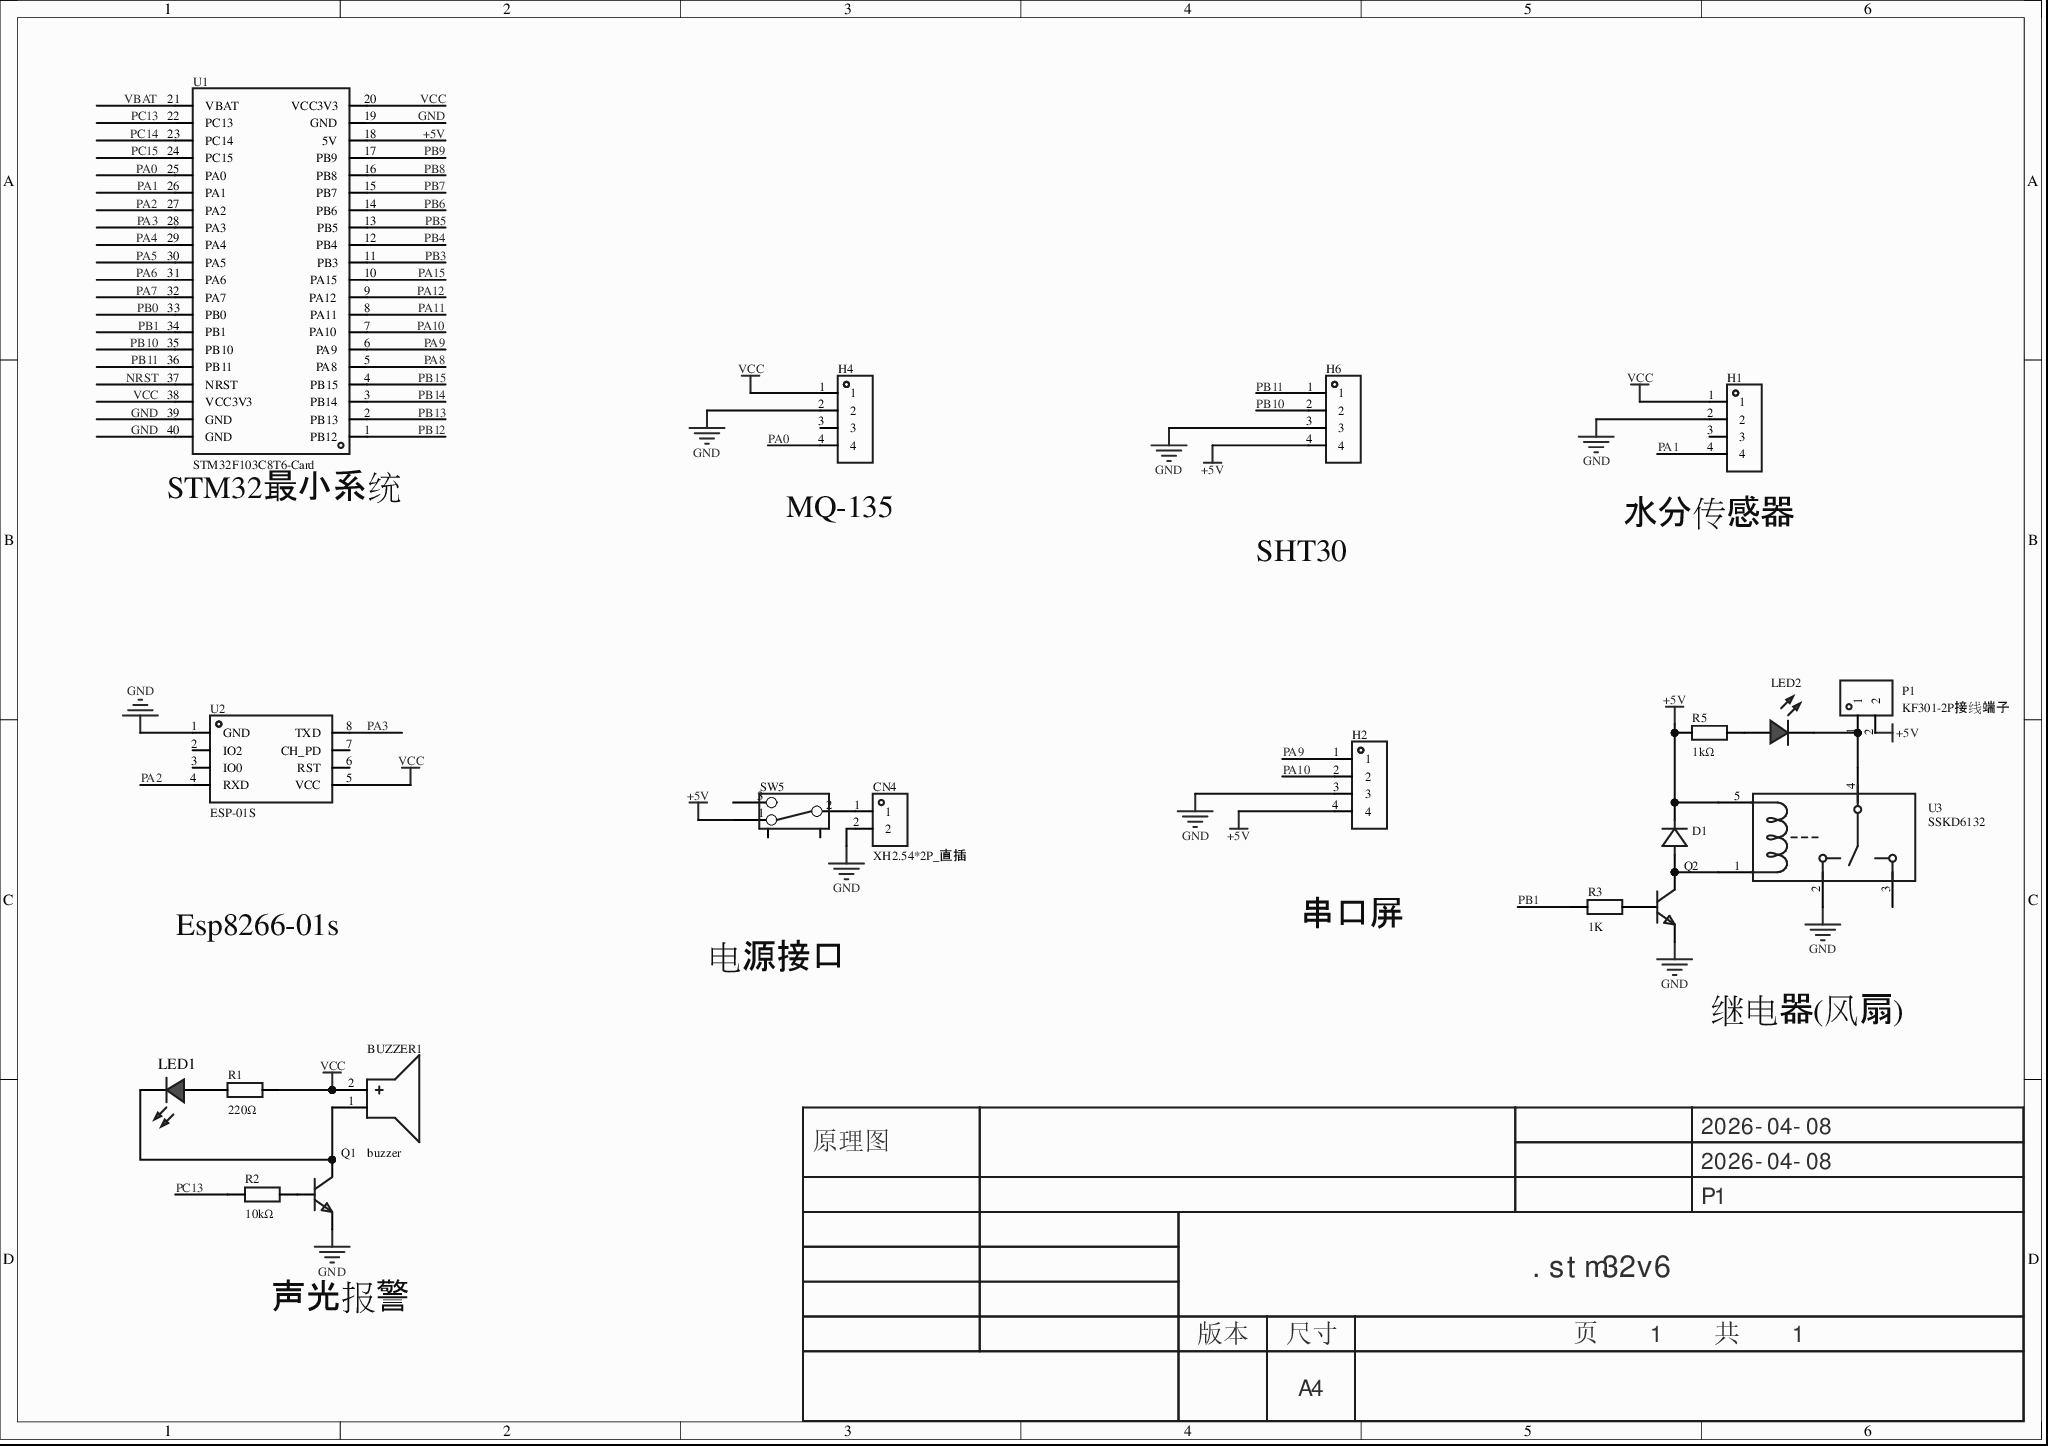
[diagram p0: MISC52093-3.schdoc]
# Altium project MISC52093-2.PrjPcb
1 sheet, 20 parts. Net scope: global (net labels, ports and power ports of the same name join across sheets).
Board file: MISC52093.pcbdoc

## Sheet MISC52093-3.schdoc
size 297 x 209 mm; Version: V1.0; @Project Name: MISC52093; @Page Count: 1; @Update Date: 2026-04-08; @Create Date: 2026-04-08; @Schematic Name: MISC52093; @Page No: 1; @Create Time: 23:22:16; @Update Time: 17:32:40; @Board Name: MISC52093

### Parts
BUZZER1  buzzer  [BUZ-TH_BD12.0-P6.00-D0.9-RD]
CN4  XH2.54*2P_直插  [CONN-TH_2P-P2.50-XH2.54-2P]
D1  (no value)  [SMA_1N4007]
H1  (no value)  [HDR-TH_4P-P2.54-V-F]
H2  (no value)  [HDR-TH_4P-P2.54-V-F]
H4  (no value)  [HDR-TH_4P-P2.54-V-F]
H6  (no value)  [HDR-TH_4P-P2.54-V-F]
LED1  (no value)  [LED_0603]
LED2  (no value)  [LED_TH-3mm]
P1  KF301-2P接线端子  [CONN-TH_XY301V-A-5.0-2P]
Q1  (no value)  [S8050_TO_92]
Q2  (no value)  [S8050_SOT-23]
R1  220Ω  [Res_1/8W]
R2  10kΩ  [Res_1/8W]
R3  1K  [R0603]
R5  1kΩ  [Res_1/8W]
SW5  (no value)  [拨动开关]
U1  STM32F103C8T6-Card  [CONN-TH_L53.3-W22.9_STM32F103C8T6-CARD]
U2  ESP-01S  [WIFIM-TH_ESP-01S]
U3  SSKD6132  [RELAY-TH_G2R-1]

### Nets
+5V: D1.1(K) H2.4 H6.4 P1.2 R5.1 SW5.1 U1.18(5V) U3.5
GND: CN4.2 H1.2 H2.3 H4.2 H6.3 Q1.1(E) Q2.2 U1.19(GND) U1.39(GND) U1.40(GND) U2.1(GND) U3.2
VCC: BUZZER1.2(+) H1.1 H4.1 R1.2 U1.20(VCC3V3) U1.38(VCC3V3) U2.5(VCC)
NRST: U1.37(NRST)
PA0: H4.4 U1.25(PA0)
PA1: H1.4 U1.26(PA1)
PA2: U1.27(PA2) U2.4(RXD)
PA3: U1.28(PA3) U2.8(TXD)
PA4: U1.29(PA4)
PA5: U1.30(PA5)
PA6: U1.31(PA6)
PA7: U1.32(PA7)
PA8: U1.5(PA8)
PA9: H2.1 U1.6(PA9)
PA10: H2.2 U1.7(PA10)
PA11: U1.8(PA11)
PA12: U1.9(PA12)
PA15: U1.10(PA15)
PB0: U1.33(PB0)
PB1: R3.1 U1.34(PB1)
PB3: U1.11(PB3)
PB4: U1.12(PB4)
PB5: U1.13(PB5)
PB6: U1.14(PB6)
PB7: U1.15(PB7)
PB8: U1.16(PB8)
PB9: U1.17(PB9)
PB10: H6.2 U1.35(PB10)
PB11: H6.1 U1.36(PB11)
PB12: U1.1(PB12)
PB13: U1.2(PB13)
PB14: U1.3(PB14)
PB15: U1.4(PB15)
PC13: R2.1 U1.22(PC13)
PC14: U1.23(PC14)
PC15: U1.24(PC15)
VBAT: U1.21(VBAT)
NetBUZZER1_1: BUZZER1.1(-) LED1.1(C) Q1.3(C)
NetCN4_1: CN4.1 SW5.2
NetD1_2: D1.2(A) Q2.3 U3.1
NetLED1_2: LED1.2(A) R1.1
NetLED2_1: LED2.1(C) R5.2
NetLED2_2: LED2.2(A) P1.1 U3.4
NetQ1_2: Q1.2(B) R2.2
NetQ2_1: Q2.1 R3.2

Not connected (* = marked no-connect by the designer): H1 3; H4 3; SW5 3 4 5; U2 2(IO2)* 3(IO0)* 6(RST)* 7(CH_PD)*; U3 3

### Notes on the sheet
- (near U1) STM32最小系统
- (near H4) MQ-135
- SHT30
- (near H1) 水分传感器
- Esp8266-01s
- 串口屏
- 电源接口
- 继电器(风扇)
- 声光报警
- Labels drawn without touching a wire or pin: VCC
- 2026-04-08
- 原理图
- P1
- .stm32v6
- 版本
- 尺寸
- A4
- 页    1    共    1

### Library data of the parts
BUZZER1 = buzzer: 3D Model: af17e4151ed84fc2a628230bf23763630819f05c4eef4c71ace90d822a990e87; 3D Model Transform: 472.44,472.176,0,270,0,0,0,0,-196.85; AddInBom: yes; Symbol: BUZZER; Device: buzzer; LCSC Part Name: buzzer; Supplier Part: C9900014030; Manufacturer Part: buzzer; Supplier Footprint: buzzer; JLCPCB Part Class: Extended Part; Supplier: LCSC; ConvertToPcb: yes; FootprintName: BUZ-TH_BD12.0-P6.00-D0.9-RD; ModelName: BUZ-TH_BD12.0-P6.00-D0.9-RD
CN4 = XH2.54*2P_直插: 3D Model: 325c595e30db4df8abe76612dd40b0fa0819f05c4eef4c71ace90d822a990e87; 3D Model Transform: 295.275,228.346,0,180,0,0,-0.002,-20.079,-137.795; AddInBom: yes; Symbol: XH2.54*2P_直插; Device: XH2.54*2P_直插; LCSC Part Name: XH2.54*2P_直插; Supplier Part: C9900008615; Manufacturer Part: XH2.54*2P_直插; Supplier Footprint: XH2.54_2P; JLCPCB Part Class: Extended Part; Supplier: LCSC; ConvertToPcb: yes; FootprintName: CONN-TH_2P-P2.50-XH2.54-2P; ModelName: CONN-TH_2P-P2.50-XH2.54-2P
D1 = D_1N4007: 3D Model: 4f1e9ef2303f48b48aa8ce0cacf8d7b10819f05c4eef4c71ace90d822a990e87; 3D Model Transform: 204.7,102.4,82.7,0,0,0,0,0,0; AddInBom: yes; ModelName: SMA_L4.4-W2.8-LS5.4-RD; Symbol: D_1N4007; Device: D_1N4007; Supplier Footprint: SMA; ConvertToPcb: yes; FootprintName: SMA_1N4007
H1 H2 H4 H6 = HDR-F_2.54_1x4P: Symbol: 2.54-1*4P母; 3D Model: d187812051054f85879fcaa51a310d8e0819f05c4eef4c71ace90d822a990e87; 3D Model Transform: 419.6842,98.464,0,0,0,0,0,0,-118.11; ConvertToPcb: yes; Device: HDR-F_2.54_1x4P; Supplier Part: C2718488; Supplier Footprint: 插件; FootprintName: HDR-TH_4P-P2.54-V-F; AddInBom: yes; ModelName: HDR-TH_4P-P2.54-V-F
LED1 = LED_0603-R: Symbol: LED_R; Convert to PCB: yes; 3D Model: dd8257b0d61a4cd7b68939a056e08095; 3D Model Transform: 58.72,29.4,22.03,0,0,0,0,0,0; ModelName: LED-0603_R; Device: LED_0603-R; Add into BOM: yes; Supplier Footprint: 0603; FootprintName: LED_0603
LED2 = LED_TH-R_3mm: 3D Model: a497c992633541038a38947cdc58012f0819f05c4eef4c71ace90d822a990e87; 3D Model Transform: 141.274,153.327,0,0,0,0,-5.984,0,-137.795; ConvertToPcb: yes; ModelName: LED-TH-3mm_R; Symbol: LED_TH-R; Device: LED_TH-R_3mm; Supplier Footprint: 插件; AddInBom: yes; FootprintName: LED_TH-3mm
P1 = KF301-2P接线端子: 3D Model: ef7ead88b0f2448d904975b26718870f; 3D Model Transform: 417.322,299.212,0,0,0,0,11.811,-7.835,-157.48; AddInBom: yes; Symbol: KF301-2P接线端子; Device: KF301-2P接线端子; LCSC Part Name: KF301-2P接线端子; Supplier Part: C9900016950; Manufacturer Part: KF301-2P接线端子; Supplier Footprint: CK301-2P; Supplier: LCSC; ConvertToPcb: yes; FootprintName: CONN-TH_XY301V-A-5.0-2P; ModelName: CONN-TH_XY301V-A-5.0-2P
Q1 = S8050_TO_NPN: 3D Model: aafe8e06f2154e7c93506efd0d6632dd; 3D Model Transform: 180.78,141.44,417.3,0,0,0,0,0,-200; ConvertToPcb: yes; ModelName: TO-92-3_L4.9-W3.7-P1.27-L; Symbol: S8050_TO_NPN; Device: S8050_TO_NPN; Supplier Footprint: TO-92; AddInBom: yes; FootprintName: S8050_TO_92
Q2 = S8050_SOT_NPN: Symbol: NPN; 3D Model: c62791f0466c4ae2a892c056b845b0ca0819f05c4eef4c71ace90d822a990e87; 3D Model Transform: 98.6,114.12,41.29,180,0,0,0,0,-3; ConvertToPcb: yes; ModelName: SOT-23-3P_L2.9-W1.3-H1.0-LS2.4-P0.95; Device: S8050_SOT_NPN; Supplier Footprint: SOT-23; AddInBom: yes; FootprintName: S8050_SOT-23
R1 R2 R5 = Res_AXIAL-1/8W: Symbol: 电阻; 3D Model: b2b5ae7ae4c642178fe0039925c86a3f; 3D Model Transform: 282.86,66.88,253.09,0,0,0,0,0,-191; ConvertToPcb: yes; ModelName: RES-TH_BD1.8-L3.2-P7.20-D0.4; Device: Res_AXIAL-1/8W; Supplier Footprint: 轴向引线; AddInBom: yes; FootprintName: Res_1/8W
  R1: Value: 220Ω
  R2: Value: 10kΩ
  R5: Value: 1kΩ
R3 = Res_0603: Symbol: 电阻; 3D Model: fc143cca1e79419f9cd78b61e9279f080819f05c4eef4c71ace90d822a990e87; 3D Model Transform: 31.8897,63.7794,0,90,0,0,0,0,0; ConvertToPcb: yes; Device: Res_0603; Value: 1K; Supplier Footprint: 0603; AddInBom: yes; FootprintName: R0603; ModelName: R0603
SW5 = 拨动开关_正: ConvertToPcb: yes; ModelId: 4321fe59a4074cbfb4989553f297c68f0819f05c4eef4c71ace90d822a990e87; ModelName: SW-TH_SS-12D02-VG4; ModelTransform: 370.09,208.7,472.35,0,0,0,0,0,-110; Symbol: 拨动开关; Device: 拨动开关_正; AddInBom: yes; Supplier Footprint: 插件; FootprintName: 拨动开关
U1 = STM32F103C8T6-Card: AddInBom: yes; Symbol: STM32F103C8T6-CARD; Device: STM32F103C8T6-Card; LCSC Part Name: STM32F103C8T6-Card; SupplierPart: C9900077949; ManufacturerPart: STM32F103C8T6-Card; Supplier Footprint: 插件; Supplier: LCSC; ConvertToPcb: yes; FootprintName: CONN-TH_L53.3-W22.9_STM32F103C8T6-CARD
U2 = ESP-01S_C111009: AddInBom: yes; ModelId: eb7175da78ae48b3b1568cfe3027405f0819f05c4eef4c71ace90d822a990e87; ModelTransform: 582.676,976.37608,0,0,0,0,0,388.346,-118.11; Symbol: ESP-01S; Device: ESP-01S_C111009; LCSC Part Name: ESP-01S; SupplierPart: C111009; ManufacturerPart: ESP-01S; Supplier Footprint: -; JLCPCB Part Class: Extended Part; Supplier: LCSC; ConvertToPcb: yes; FootprintName: WIFIM-TH_ESP-01S; ModelName: WIFIM-TH_ESP-01S
U3 = SSKD6132: 3D Model: fe99462dd15043c98af5adb0e5338dda0819f05c4eef4c71ace90d822a990e87; 3D Model Transform: 1141.73,511.81,0,0,0,0,26.417,-0.354,-157.48; AddInBom: yes; Symbol: SSKD6132; Device: SSKD6132; LCSC Part Name: SSKD6132; Supplier Part: C9900012103; Manufacturer Part: SSKD6132; Supplier Footprint: RELAY-TH_G2R-1; JLCPCB Part Class: Extended Part; Supplier: LCSC; ConvertToPcb: yes; FootprintName: RELAY-TH_G2R-1; ModelName: RELAY-TH_G2R-1